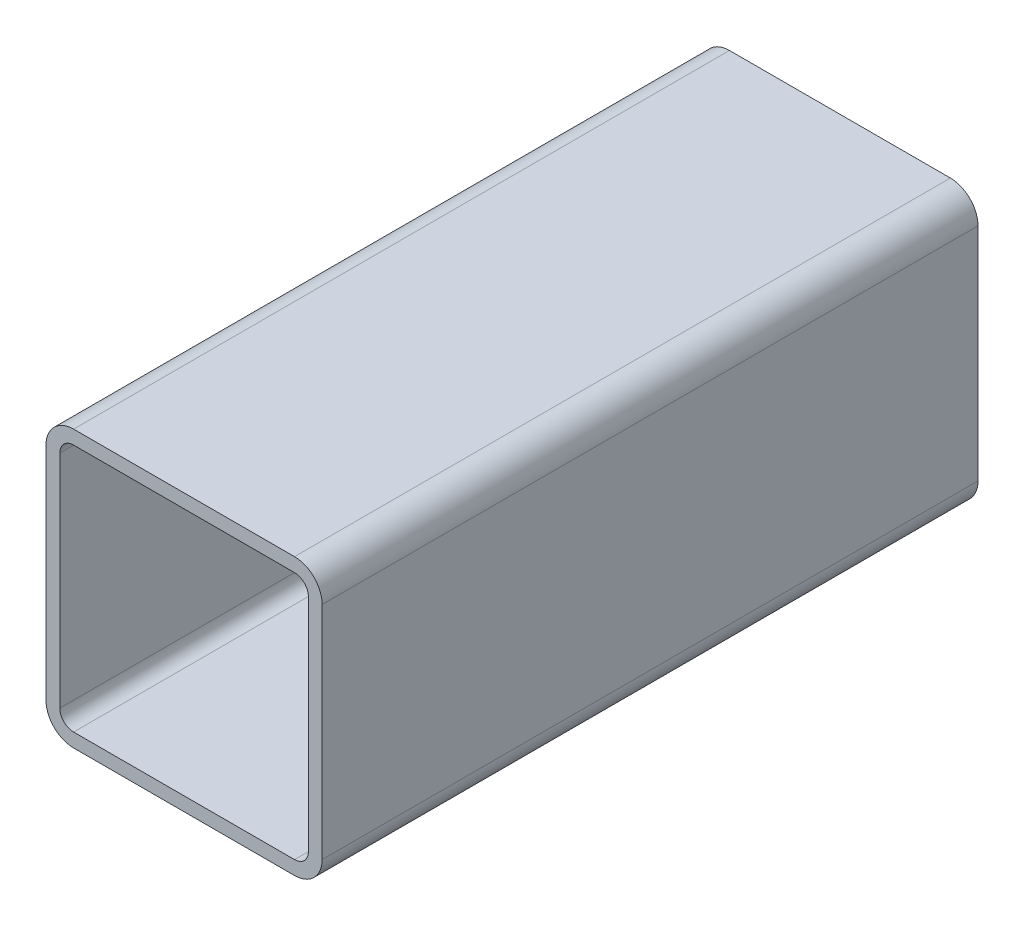
SolidWorks part; units mm, degrees
material "Q235A"
ref_plane "Front Plane" through (0, 0, 0) normal (0, 0, 1) x (1, 0, 0)
ref_plane "Top Plane" through (0, 0, 0) normal (0, 1, 0) x (1, 0, 0)
ref_plane "Right Plane" through (0, 0, 0) normal (1, 0, 0) x (0, 0, -1)
sketch "Sketch1" plane through (0, 0, 0) normal (0, 0, 1) x (1, 0, 0)
  line L1 (-20, 20) -> (20, 20)
  line L2 (-20, 20) -> (-20, -20)
  line L3 (-20, -20) -> (20, -20)
  line L4 (20, 20) -> (20, -20)
  line L5 (-20, 20) -> (20, -20) construction
  line L6 (-20, -20) -> (20, 20) construction
  line L7 (-18, 18) -> (18, 18)
  line L8 (-18, 18) -> (-18, -18)
  line L9 (-18, -18) -> (18, -18)
  line L10 (18, 18) -> (18, -18)
  line L11 (-18, 18) -> (18, -18) construction
  line L12 (-18, -18) -> (18, 18) construction
  point P0 (0, 0)
  point P6 (0, 0)
  dimension "D1" = 40
  dimension "D2" = 40
  dimension "D3" = 2
  dimension "D4" = 2
extrude "Boss-Extrude1" add sketch "Sketch1" along normal blind 95
fillet "Fillet1" radius 2 4 edges at (18, 18, 47.5) (-18, 18, 47.5) (-18, -18, 47.5) (18, -18, 47.5)
fillet "Fillet2" radius 4 4 edges at (20, 20, 47.5) (20, -20, 47.5) (-20, 20, 47.5) (-20, -20, 47.5)
